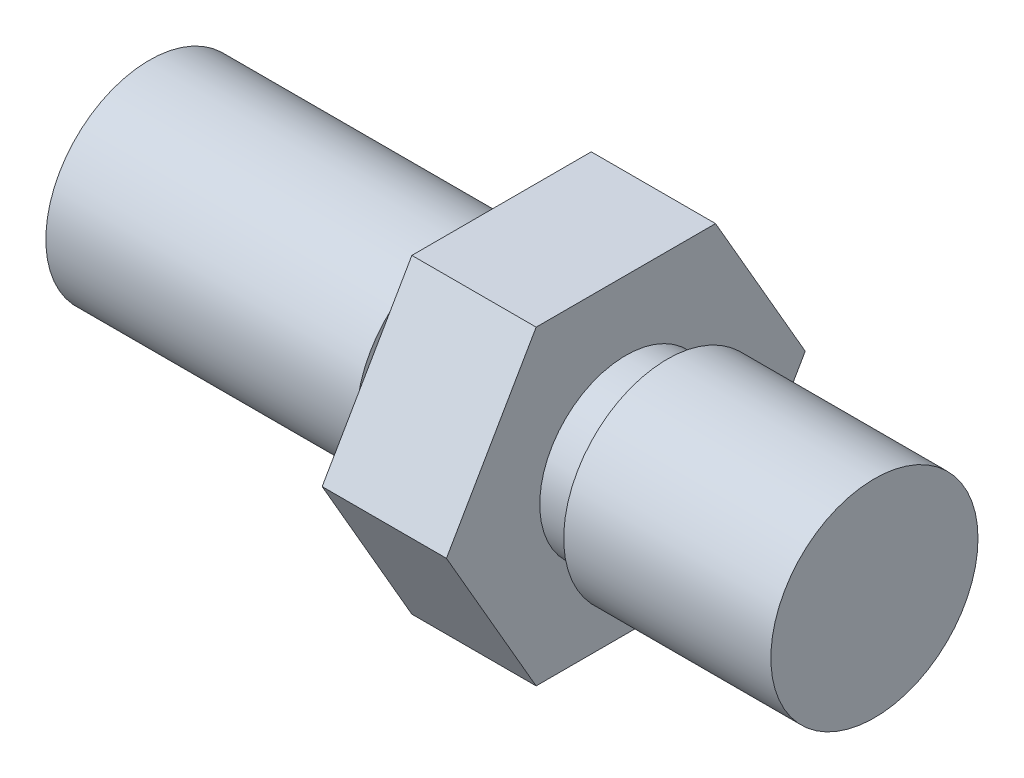
SolidWorks part; units mm, degrees
ref_plane "前视基准面" through (0, 0, 0) normal (0, 0, 1) x (1, 0, 0)
ref_plane "上视基准面" through (0, 0, 0) normal (0, 1, 0) x (1, 0, 0)
ref_plane "右视基准面" through (0, 0, 0) normal (1, 0, 0) x (0, 0, -1)
ref_plane "基准面4" through (8, 0, 0) normal (1, 0, 0) x (0, 0, -1)
sketch "草图1" plane through (8, 0, 0) normal (1, 0, 0) x (0, 0, -1)
  line L0 (-8.6603, 0) -> (-4.3301, -7.5)
  line L1 (-4.3301, -7.5) -> (4.3301, -7.5)
  line L2 (4.3301, -7.5) -> (8.6603, 0)
  line L3 (8.6603, 0) -> (4.3301, 7.5)
  line L4 (4.3301, 7.5) -> (-4.3301, 7.5)
  line L5 (-4.3301, 7.5) -> (-8.6603, 0)
extrude "凸台-拉伸1" add sketch "草图1" against normal blind 6
sketch "草图2" plane through (0, 0, 0) normal (0, 0, 1) x (1, 0, 0)
  line L0 (-15, 5) -> (-15, 0)
  line L1 (-15, 0) -> (2, 0)
  line L2 (2, 0) -> (2, 4.1572)
  line L3 (2, 4.1572) -> (0, 4.1572)
  line L4 (0, 4.1572) -> (0, 5)
  line L5 (0, 5) -> (-15, 5)
  line L6 (-15, 0) -> (2, 0) construction
revolve "旋转1" add sketch "草图2" angle 360 about L6
sketch "草图3" plane through (0, 0, 0) normal (0, 0, 1) x (1, 0, 0)
  line L0 (8, 4.1572) -> (8, 0)
  line L1 (8, 0) -> (20, 0)
  line L2 (20, 0) -> (20, 5)
  line L3 (20, 5) -> (10, 5)
  line L4 (10, 5) -> (10, 4.1572)
  line L5 (10, 4.1572) -> (8, 4.1572)
  line L6 (8, 0) -> (20, 0) construction
revolve "旋转2" add sketch "草图3" angle 360 about L6
